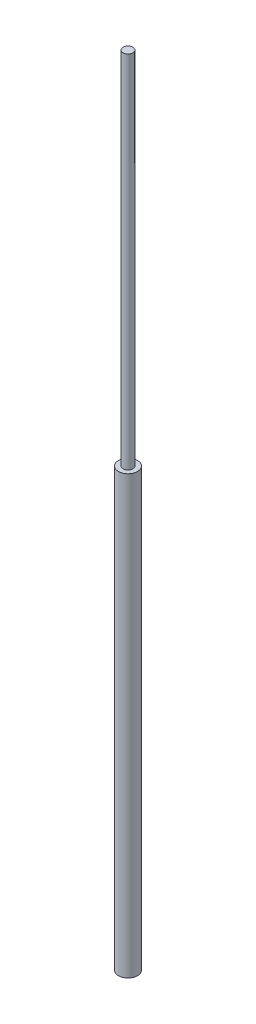
from build123d import *

# Parameters (mm, degrees)
SKETCH1_R           = 0.875
BOSS_EXTRUDE1_DEPTH = 40
SKETCH2_R           = 0.45
BOSS_EXTRUDE2_DEPTH = 33


with BuildPart() as part:
    # Sketch1 → Boss-Extrude1 (new body)
    with BuildSketch(Plane(origin=(0, 0, 0), x_dir=(1, 0, 0), z_dir=(0, 1, 0))):
        with Locations(Location((0, 0, 0), (0, 0, 270))):
            Circle(SKETCH1_R)
    extrude(amount=BOSS_EXTRUDE1_DEPTH)

    # Sketch2 → Boss-Extrude2 (add)
    with BuildSketch(Plane(origin=(0, 40, 0), x_dir=(1, 0, 0), z_dir=(0, 1, 0))):
        with Locations(Location((0, 0, 0), (0, 0, 270))):
            Circle(SKETCH2_R)
    extrude(amount=BOSS_EXTRUDE2_DEPTH)


solid = part.part
